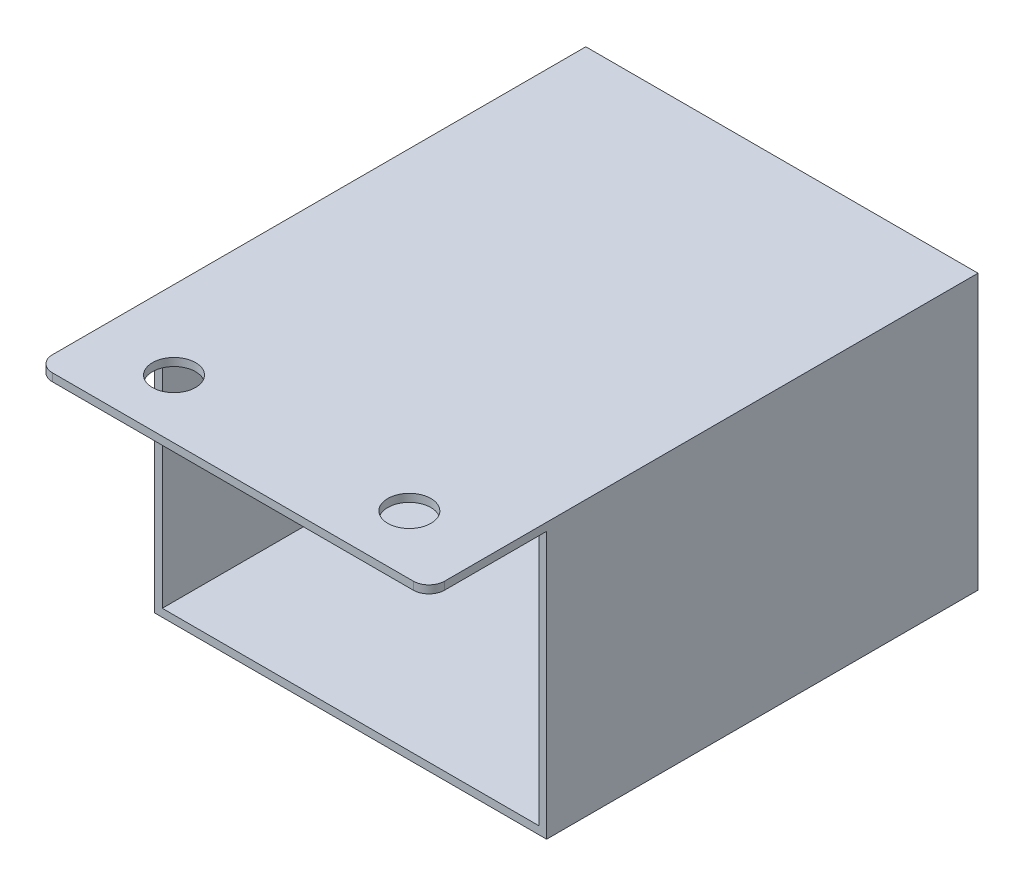
from build123d import *

# Parameters (mm, degrees)
SKETCH_1_W          = 50
SKETCH_1_H          = 35
EXTRUDE_1_DEPTH     = 55
SKETCH_2_W          = 48
SKETCH_2_H          = 33
CUT_EXTRUDE_1_DEPTH = 54
SKETCH_5_W          = 50
SKETCH_5_H          = 1
EXTRUDE_2_DEPTH     = 15
SKETCH_6_R          = 2.75
CUT_EXTRUDE_3_DEPTH = 12
FILLET_1_R          = 2


with BuildPart() as part:
    # 草图1 → 凸台-拉伸1 (new body)
    with BuildSketch(Plane.XY):
        Rectangle(SKETCH_1_W, SKETCH_1_H)
    extrude(amount=EXTRUDE_1_DEPTH)

    # 草图2 → 切除-拉伸1 (cut)
    with BuildSketch(Plane.XY.offset(55)):
        Rectangle(SKETCH_2_W, SKETCH_2_H)
    extrude(amount=-CUT_EXTRUDE_1_DEPTH, mode=Mode.SUBTRACT)

    # 草图5 → 凸台-拉伸2 (add)
    with BuildSketch(Plane.XY.offset(55)):
        with Locations((0, 17)):
            Rectangle(SKETCH_5_W, SKETCH_5_H)
    extrude(amount=EXTRUDE_2_DEPTH)

    # 草图6 → 切除-拉伸3 (cut)
    with BuildSketch(Plane.XZ.offset(-16.5)):
        with Locations(Location((-15, 62.5, 0), (0, 0, 270))):
            Circle(SKETCH_6_R)
        with Locations(Location((15, 62.5, 0), (0, 0, 270))):
            Circle(SKETCH_6_R)
    extrude(amount=-CUT_EXTRUDE_3_DEPTH, mode=Mode.SUBTRACT)

    # 圆角1
    fillet_1_edges = [part.edges().sort_by_distance(p)[0] for p in [
        (25, 17, 70),
        (-25, 17, 70),
    ]]
    fillet(fillet_1_edges, radius=FILLET_1_R)


solid = part.part
